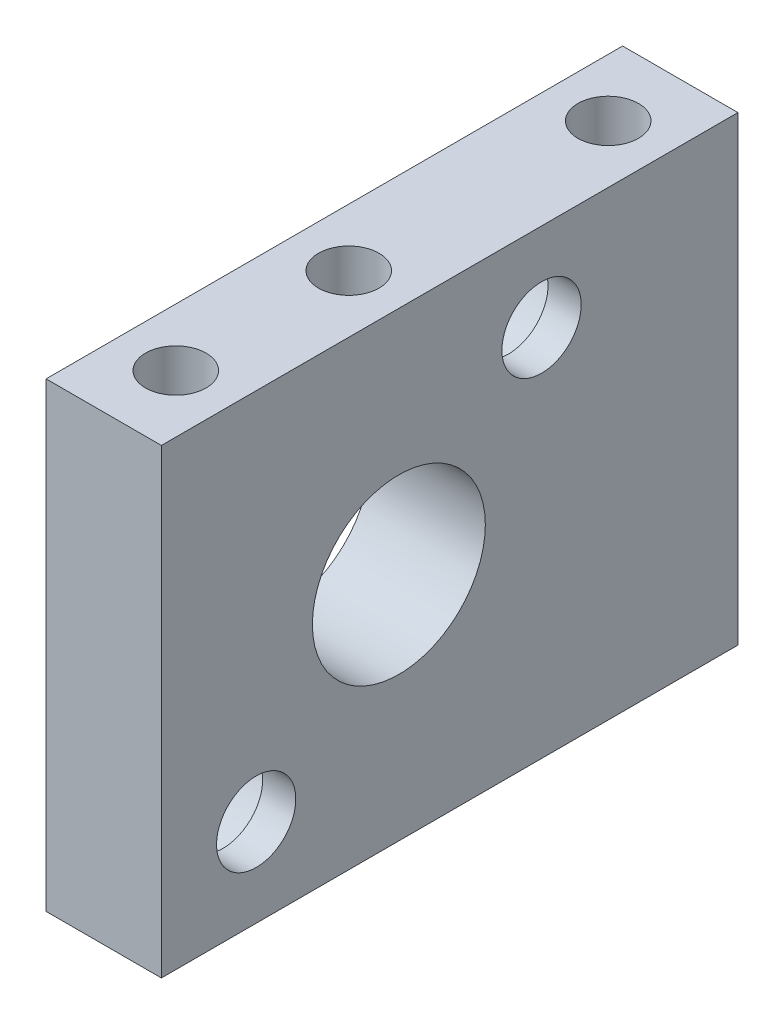
from build123d import *

# Parameters (mm, degrees)
SKETCH_1_W                = 40
SKETCH_1_H                = 32
EXTRUDE_1_DEPTH           = 8
SKETCH_8_R                = 6
CUT_EXTRUDE_2_DEPTH       = 27.83281573
HOLE_WIZARD_3_D           = 5.5
HOLE_WIZARD_3_CBORE_D     = 10
HOLE_WIZARD_3_CBORE_DEPTH = 5.7
HOLE_WIZARD_M5_1_D        = 4.2
HOLE_WIZARD_M5_1_DEPTH    = 12.4
HOLE_WIZARD_M5_1_TIP      = 1.2618073


with BuildPart() as part:
    # 草图1 → 凸台-拉伸1 (new body)
    with BuildSketch(Plane(origin=(0, 0, 0), x_dir=(0, 0, -1), z_dir=(1, 0, 0))):
        Rectangle(SKETCH_1_W, SKETCH_1_H)
    extrude(amount=EXTRUDE_1_DEPTH)

    # 草图8 → 切除-拉伸2 (cut, through all)
    with BuildSketch(Plane.ZY):
        with Locations((3.523652159, 0)):
            Circle(SKETCH_8_R)
    extrude(amount=-CUT_EXTRUDE_2_DEPTH, mode=Mode.SUBTRACT)

    # 打孔尺寸(%根据)内六角圆柱头螺钉的类型3 (through all)
    with Locations(Plane.ZY):
        with Locations((-6.375842777, 9.899494937), (13.423147096, -9.899494937)):
            CounterBoreHole(HOLE_WIZARD_3_D / 2, HOLE_WIZARD_3_CBORE_D / 2, HOLE_WIZARD_3_CBORE_DEPTH)

    # M5 螺纹孔1
    with Locations(Plane(origin=(0, 16, 0), x_dir=(1, 0, 0), z_dir=(0, 1, 0))):
        with Locations((4, -3), (4, -15), (4, 15)):
            Hole(HOLE_WIZARD_M5_1_D / 2, depth=HOLE_WIZARD_M5_1_DEPTH)
            with Locations((0, 0, -(HOLE_WIZARD_M5_1_DEPTH + HOLE_WIZARD_M5_1_TIP / 2))):  # 118° drill point
                Cone(0, HOLE_WIZARD_M5_1_D / 2, HOLE_WIZARD_M5_1_TIP, mode=Mode.SUBTRACT)


solid = part.part
